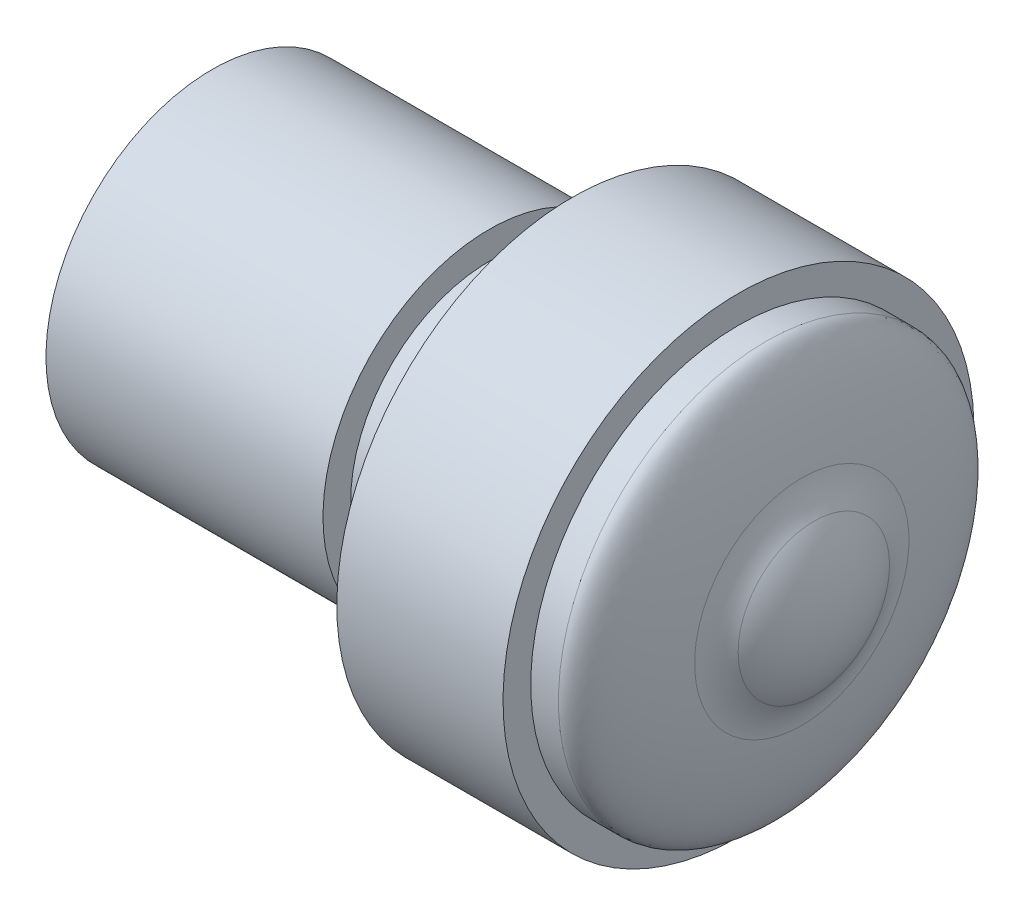
SolidWorks part; units mm, degrees
ref_plane "Front Plane" through (0, 0, 0) normal (0, 0, 1) x (1, 0, 0)
ref_plane "Top Plane" through (0, 0, 0) normal (0, 1, 0) x (1, 0, 0)
ref_plane "Right Plane" through (0, 0, 0) normal (1, 0, 0) x (0, 0, -1)
sketch "Sketch1" plane through (0, 0, 0) normal (0, 0, 1) x (1, 0, 0)
  line L0 (0, 0) -> (45.4931, 0) construction
  line L1 (0, 0) -> (0, 12)
  line L2 (0, 12) -> (20, 12)
  line L3 (20, 12) -> (20, 10)
  line L4 (20, 10) -> (25.9985, 10)
  line L5 (25.9985, 10) -> (25.9985, 17)
  line L6 (25.9985, 17) -> (37.9985, 17)
  line L7 (37.9985, 17) -> (37.9985, 15)
  line L8 (37.9985, 15) -> (39.9985, 15)
  line L9 (39.9985, 15) -> (39.9985, 0) construction
  line L10 (0, 0) -> (45, 0)
  arc A0 (43.4385, 5.4657) -> (42.5685, 7.7381) centre (47.5326, 8.3359) cw
  ellipse E0 centre (39.9985, 0) end of major axis (39.9985, -15) minor radius 3 (42.5685, 7.7381) -> (39.9985, 15) ccw
  ellipse E2 centre (39.9985, 0) end of major axis (39.9985, 7.5295) minor radius 5.0015 (45, 0) -> (43.4385, 5.4657) ccw
  dimension "D12" = 5
  dimension "D1" = 12
  dimension "D2" = 20
  dimension "D3" = 12
  dimension "D4" = 10
  dimension "D5" = 17
  dimension "D6" = 2
  dimension "D7" = 15
  dimension "D8" = 5.44
  dimension "D9" = 4.57
  dimension "D10" = 45
  dimension "D11" = 3
revolve "Revolve1" add sketch "Sketch1" angle 360 about L10
